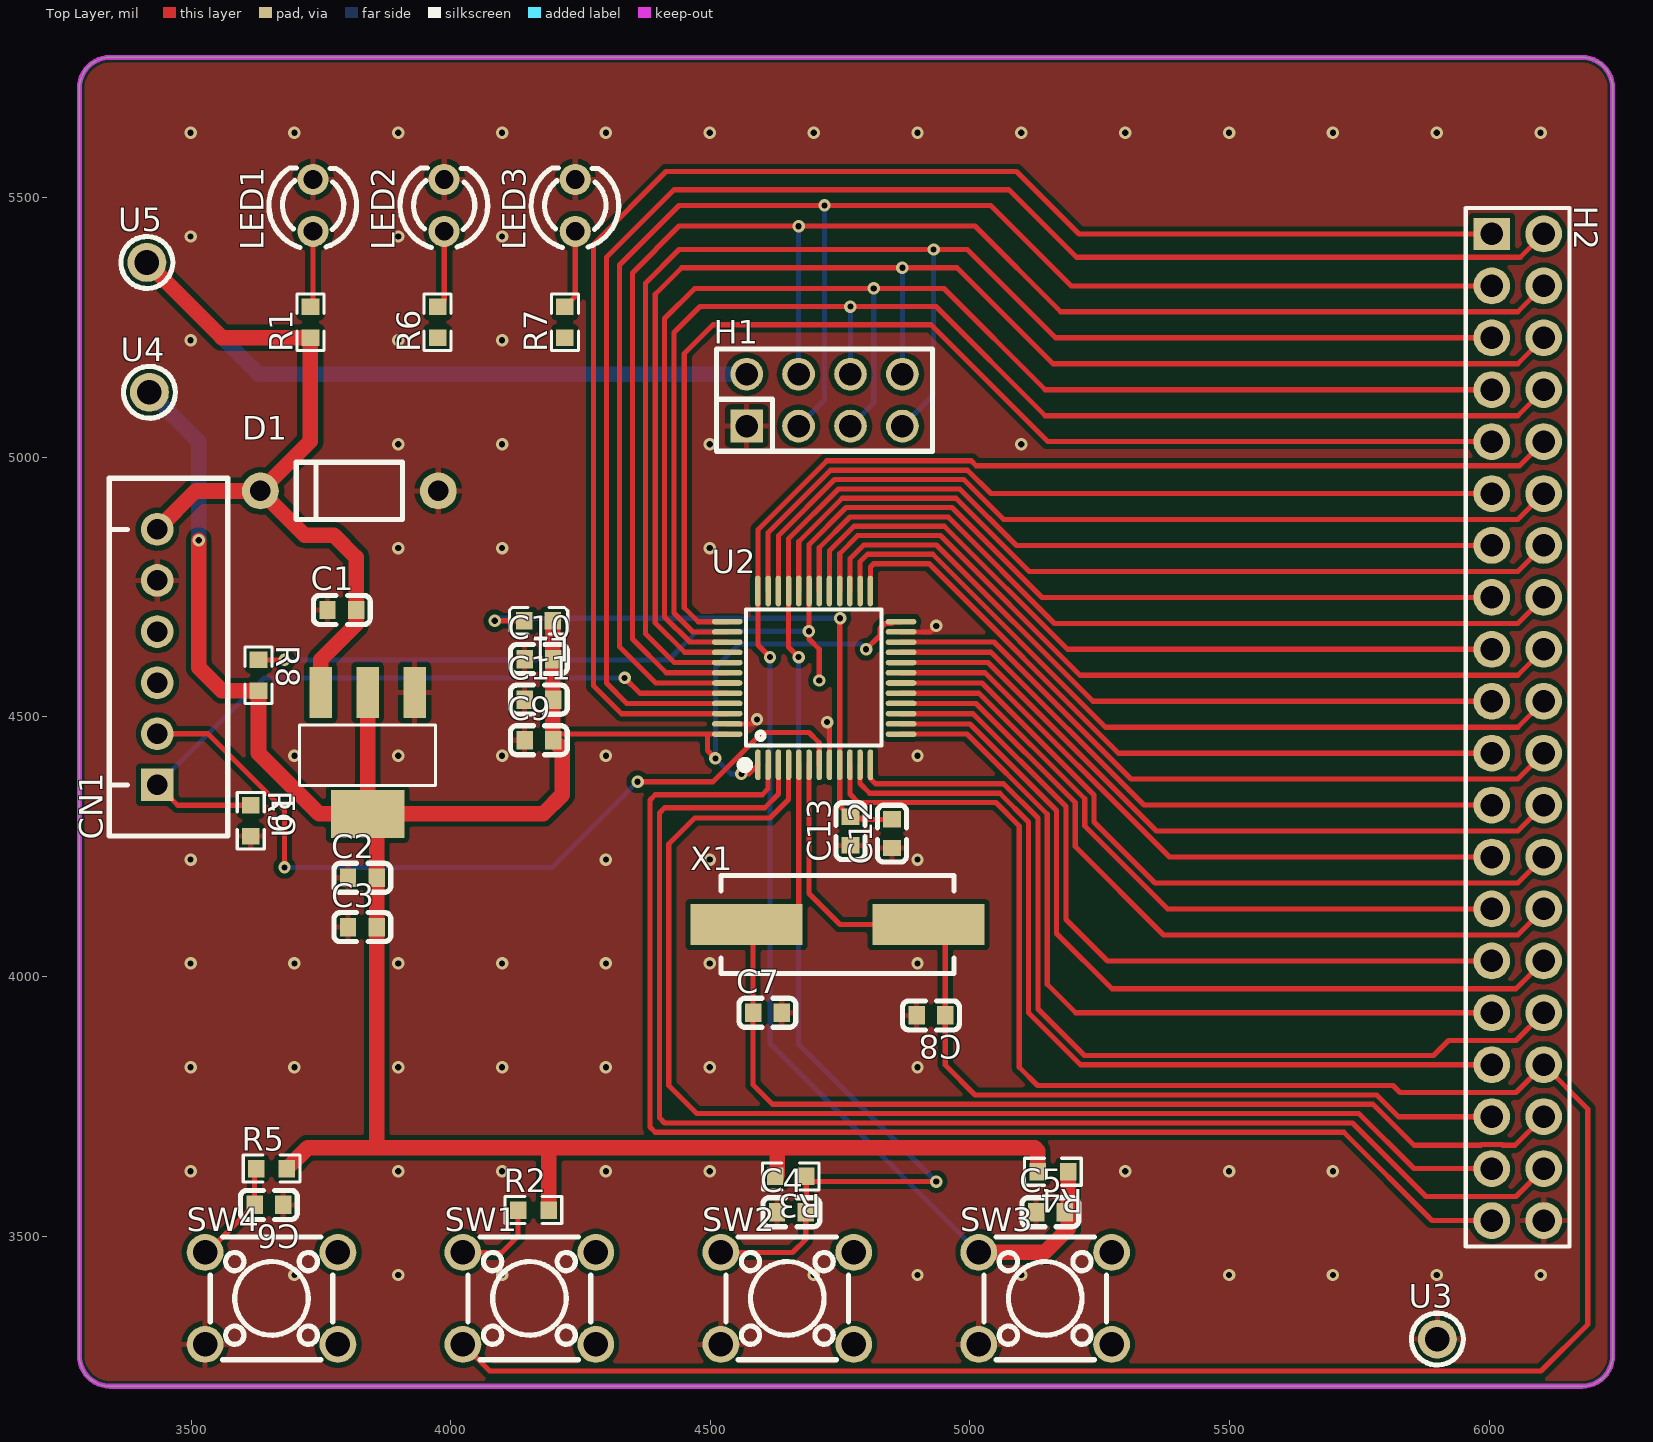
[diagram p0: Top Layer view]
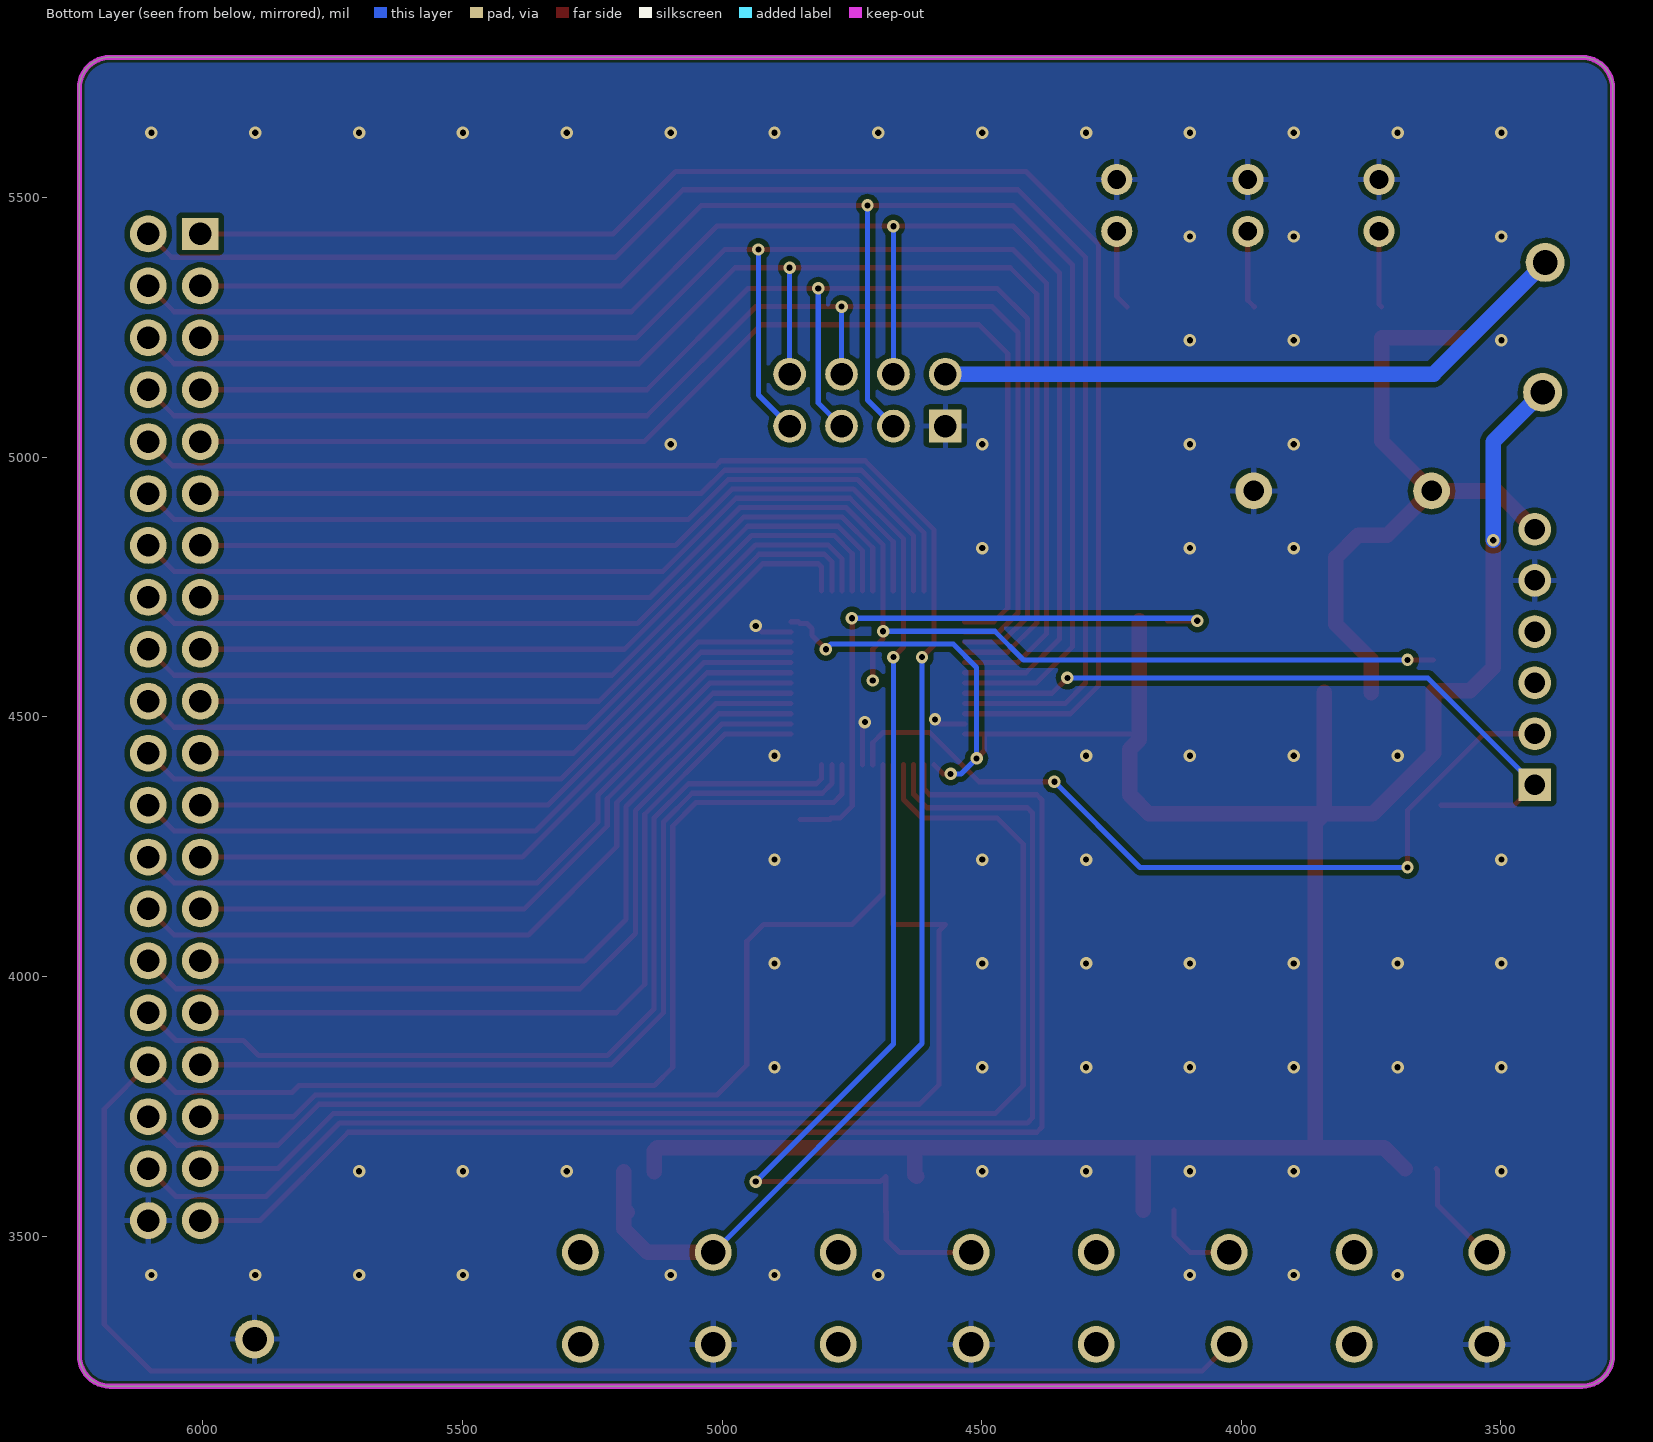
[diagram p1: Bottom Layer view, seen from below]
# Altium PCB MISC75379.pcbdoc
Units mil, origin at the board's own origin, x right, y up, seen from the top; angles counter-clockwise.
Board outline 2952.76 x 2559.06 mil, 2 copper layers (Top Layer, Bottom Layer), stack 62.206 mil thick; 40 components, 54 nets, 181 pads, 92 vias.

## Layer stack, top to bottom
Top Solder Mask Layer: solder mask 0.394, Dk 3.3
Top Layer: signal copper 1.379
Dielectric1: surface 59.449, FR4, Dk 4.5
Bottom Layer: signal copper 1.378
Bottom Solder Mask Layer: solder mask 0.394, Dk 3.3

## Board outline
3344.06,5770 ccw(c3344.06,5710.94) 3285,5710.94 3285,3270 ccw(c3344.06,3270) 3344.06,3210.94 6178.7,3210.94 ccw(c6178.7,3270) 6237.76,3270 6237.76,5710.94 ccw(c6178.7,5710.94) 6178.7,5770 3344.06,5770

## Design rules (kind name [scope] priority, off if disabled: settings)
BoardOutlineClearance copperThickness2oz_1 [All] p2 off: genericclearance=7.99 ignorepadtopadclearanceinfootprint=FALSE except(0: Arc-SplitContinuation Track-SplitContinuation SMDPad-SplitContinuation THPad-SplitContinuation Via-SplitContinuation Fill-SplitContinuation Region-SplitContinuation Poly-SplitContinuation Text-SplitContinuation Hole-SplitContinuation; 5.98: Arc-CutoutEdge SMDPad-CutoutEdge THPad-CutoutEdge Via-CutoutEdge Fill-CutoutEdge Region-CutoutEdge Text-CutoutEdge; 6.93: Hole-OutlineEdge Hole-CutoutEdge; 10: Poly-OutlineEdge Poly-CutoutEdge; 11.81: Arc-OutlineEdge Track-OutlineEdge SMDPad-OutlineEdge THPad-OutlineEdge Via-OutlineEdge Fill-OutlineEdge Region-OutlineEdge Text-OutlineEdge Track-CutoutEdge)
BoardOutlineClearance copperThickness1oz_1 [All] p4: genericclearance=8 ignorepadtopadclearanceinfootprint=FALSE except(0: Arc-SplitContinuation Track-SplitContinuation SMDPad-SplitContinuation THPad-SplitContinuation Via-SplitContinuation Fill-SplitContinuation Region-SplitContinuation Poly-SplitContinuation Text-SplitContinuation Hole-SplitContinuation; 6: SMDPad-CutoutEdge THPad-CutoutEdge Via-CutoutEdge Fill-CutoutEdge Region-CutoutEdge Text-CutoutEdge; 6.93: Hole-OutlineEdge Hole-CutoutEdge; 10: Poly-OutlineEdge Poly-CutoutEdge; 11.8: Arc-OutlineEdge Track-OutlineEdge SMDPad-OutlineEdge THPad-OutlineEdge Via-OutlineEdge Fill-OutlineEdge Region-OutlineEdge Text-OutlineEdge; 11.81: Arc-CutoutEdge Track-CutoutEdge)
Clearance copperThickness2oz [All] p1 off: gap=7.99 ignorepadtopadclearanceinfootprint=FALSE except(5.98: SMDPad-Track SMDPad-SMDPad THPad-Track SMDPad-THPad THPad-THPad Track-Via SMDPad-Via THPad-Via Via-Via Fill-Track Region-Track Fill-SMDPad Region-SMDPad Fill-THPad Region-THPad Fill-Via Region-Via Fill-Fill Fill-Region Region-Region Arc-Track Arc-SMDPad Arc-THPad Arc-Via Fill-Arc Region-Arc Arc-Arc Text-Track SMDPad-Text Text-THPad Text-Via Fill-Text Region-Text Arc-Text Text-Text; 6.93: Hole-Track Hole-SMDPad Hole-THPad Hole-Via Fill-Hole Region-Hole Hole-Arc Hole-Text; 10: Poly-Track Poly-SMDPad Poly-THPad Poly-Via Poly-Fill Poly-Region Poly-Poly Poly-Arc Poly-Text Poly-Hole)
Clearance copperThickness1oz [All] p3: gap=8 ignorepadtopadclearanceinfootprint=FALSE except(5.98: SMDPad-Track SMDPad-SMDPad THPad-Track SMDPad-THPad THPad-THPad Track-Via SMDPad-Via THPad-Via Fill-Track Region-Track Fill-SMDPad Region-SMDPad Fill-THPad Region-THPad Fill-Via Region-Via; 6: Arc-Track Arc-SMDPad Arc-THPad Arc-Via Fill-Arc Region-Arc Text-Track SMDPad-Text Text-THPad Text-Via Fill-Text Region-Text Arc-Text; 6.93: Hole-Track Hole-SMDPad Hole-THPad Hole-Via Fill-Hole Region-Hole Hole-Arc Hole-Text; 10: Poly-Track Poly-SMDPad Poly-THPad Poly-Via Poly-Fill Poly-Region Poly-Arc Poly-Text Poly-Hole)
DiffPairsRouting differentialPair [All] p1: maxlimit=6 minlimit=6 mostfreqgap=6 toplayer_minwidth=5 toplayer_prefwidth=10 toplayer_maxwidth=100 toplayer_mingap=6 toplayer_prefgap=6 toplayer_maxgap=6 bottomlayer_minwidth=5 bottomlayer_prefwidth=10 bottomlayer_maxwidth=100 bottomlayer_mingap=6 bottomlayer_prefgap=6 bottomlayer_maxgap=6 maxuncoupledlength=10
HoleToHoleClearance otherClearance [All] p1: gap=11.81 allowstackedmicrovias=TRUE
Length netLength [All] p1: minlimit=0 maxlimit=0
MatchedLengths netLengthTolerance [All] p1: tolerance=1000
PasteMaskExpansion pasteMaskExpansion [All] p1: expansion=0
PlaneConnect innerPlane [All] p1: planeconnectstyle=Relief reliefexpansion=20 reliefentries=4 reliefconductorwidth=10 reliefairgap=10
PolygonConnect copperRegion [(InNet('GND'))] p1: connectstyle=Relief reliefconductorwidth=10 reliefentries=4 polygonreliefangle="90 Angle" airgapwidth=10 via.connectstyle=Relief via.reliefconductorwidth=10 via.reliefentries=4 via.polygonreliefangle="90 Angle" via.airgapwidth=10
RoutingVias viaSize [All] p1: holewidth=12.01 width=24.02 viastyle="Through Hole" minholewidth=11.81 minwidth=19.68 maxholewidth=248.03 maxwidth=393.7
SolderMaskExpansion solderMaskExpansion [IsVia] p1: expansion=-1000 istentingtop=TRUE
SolderMaskExpansion solderMaskExpansion [All] p2: expansion=2 istentingtop=FALSE
Width copperThickness2oz_2 [All] p1 off: maxlimit=100 minlimit=8 preferedwidth=10
Width copperThickness1oz_2 [All] p2: maxlimit=100 minlimit=5 preferedwidth=10

## Components (designator, comment, footprint, x,y, rotation, side; value= is the part's Value field where it differs from the comment)
C1 "47uF" C0603 3790.35,4705.85 r0 top
C2 "47uF" C0603 3830,4190 r0 top
C3 "100nF" C0603 3830,4095 r0 top
C4 "100nF" C0603 4656.14,3546.05 r0 top
C5 "100nF" C0603 5155,3546.05 r0 top
C6 "100nF" C0603 3650,3560 r180 top
C7 "22pF" C0603 4610,3930 r0 top
C8 "22pF" C0603 4925,3925 r180 top
C9 "100nF" C0603 4170,4455 r0 top
C10 "100nF" C0603 4170,4611.24 r0 top
C11 "100nF" C0603 4170,4533.12 r0 top
C12 "1uF" C0603 4850,4275 r90 top
C13 "10nF" C0603 4770,4280 r90 top
CN1 "XH-6A" CONN-TH_6P-P2.50_XH-6A 3435,4615 r90 top
D1 "" DO_1N4007 3805,4935 r0 top
H1 "A2541HWV-2x4P" HDR-TH_8P-P2.54-V-F-R2-C4-S2.54-1 4720,5110 r0 top
H2 "2.54mm 2*20P straight pin header" HDR-TH_40P-P2.54-V-M-R2-C20-S2.54 6055,4480 r270 top
L1 "CBG160808U000T" L0603 4169.34,4685 r180 top
LED1 "" LED_TH-3mm 3735,5485 r90 top
LED2 "" LED_TH-3mm 3987.5,5485 r90 top
LED3 "" LED_TH-3mm 4240,5485 r90 top
R1 "1K" R0603 3730,5260 r90 top
R2 "10K" R0603 4159.48,3550 r0 top
R3 "10K" R0603 4655,3615 r180 top
R4 "10K" R0603 5160,3623.95 r180 top
R5 "10K" R0603 3655,3630 r0 top
R6 "330" R0603 3975,5260 r90 top
R7 "330" R0603 4220,5260 r90 top
R8 "10K" R0603 3630,4580 r270 top
R9 "10K" R0603 3615,4300 r270 top
SW1 "TS-1095-A5B2-D1" SW-TH_4P-L6.0-W6.0-P4.50-LS6.5 4151.67,3380 r0 top
SW2 "TS-1095-A5B2-D1" SW-TH_4P-L6.0-W6.0-P4.50-LS6.5 4648.33,3380 r0 top
SW3 "TS-1095-A5B2-D1" SW-TH_4P-L6.0-W6.0-P4.50-LS6.5 5145,3380 r0 top
SW4 "TS-1095-A5B2-D1" SW-TH_4P-L6.0-W6.0-P4.50-LS6.5 3655,3380 r0 top
U1 "AMS1117-3.3" SOT-223-3_L6.5-W3.4-P2.30-LS7.0-BR 3840,4430 r90 top
U2 "GD32E230C8T6" LQFP-48_L7.0-W7.0-P0.50-LS9.0-BL 4700,4575 r0 top
U3 "RH-5000" TEST-TH_BD2.54-P1.4_RED 5900.31,3301.56 r0 top
U4 "RH-5000" TEST-TH_BD2.54-P1.4_RED 3420,5125 r0 top
U5 "RH-5000" TEST-TH_BD2.54-P1.4_RED 3415,5375 r0 top
X1 "8MHz" CRYSTAL-SMD_L11.5-W4.8-LS12.7 4745,4100 r0 top

## Footprints (in the part's own frame and the unit in brackets; to place one, negate y for a bottom-side part, rotate by r counter-clockwise, add the part's x,y. Pads: shape width x height; smd on the part's side, far side on the other; paste and mask are expansions set on the pad)
C0603 [mm]
  rect 0.8x0.9 smd: 1(-0.7,0) 2(0.7,0)
  silkscreen extent -1.39,-0.71 1.39,0.71
CONN-TH_6P-P2.50_XH-6A [mm]
  rect 1.6x1.6 hole 1: 1(-6.25,0)
  round 1.6 hole 1 copper offset 0,0: 2(-3.75,0) 6(6.25,0)
  round 1.6 hole 1: 3(-1.25,0) 4(1.25,0) 5(3.75,0)
  silkscreen extent -8.75,-3.45 8.75,2.35
CRYSTAL-SMD_L11.5-W4.8-LS12.7 [mm]
  rect 5.5x2 smd: 1(-4.45,0) 2(4.45,0)
  silkscreen extent -5.7,-2.4 5.7,2.4
DO_1N4007 [mm]
  round 1.8 hole 1 paste+0 mask+0.051: 1(-4.35,0) 2(4.35,0)
  silkscreen extent -2.6,-1.4 2.6,1.4
HDR-TH_8P-P2.54-V-F-R2-C4-S2.54-1 [mm]
  rect 1.6x1.6 hole 1.1: 1(-3.81,-1.27)
  round 1.6 hole 1.1: 2(-3.81,1.27) 3(-1.27,-1.27) 4(-1.27,1.27) 5(1.27,-1.27) 6(1.27,1.27) 7(3.81,-1.27) 8(3.81,1.27)
  silkscreen extent -5.28,-2.5 5.28,2.5
HDR-TH_40P-P2.54-V-M-R2-C20-S2.54 [mm]
  rect 1.575x1.8 hole 1.1: 1(-24.13,-1.27)
  round 1.8 hole 1.1: 2(-24.13,1.27) 3(-21.59,-1.27) 4(-21.59,1.27) 5(-19.05,-1.27) 6(-19.05,1.27) 7(-16.51,-1.27) 8(-16.51,1.27) 9(-13.97,-1.27) 10(-13.97,1.27) 11(-11.43,-1.27) 12(-11.43,1.27) 13(-8.89,-1.27) 14(-8.89,1.27) 15(-6.35,-1.27) 16(-6.35,1.27) 17(-3.81,-1.27) 18(-3.81,1.27) 19(-1.27,-1.27) 20(-1.27,1.27) 21(1.27,-1.27) 22(1.27,1.27) 23(3.81,-1.27) 24(3.81,1.27) 25(6.35,-1.27) 26(6.35,1.27) 27(8.89,-1.27) 28(8.89,1.27) 29(11.43,-1.27) 30(11.43,1.27) 31(13.97,-1.27) 32(13.97,1.27) 33(16.51,-1.27) 34(16.51,1.27) 35(19.05,-1.27) 36(19.05,1.27) 37(21.59,-1.27) 38(21.59,1.27) 39(24.13,-1.27) 40(24.13,1.27)
  silkscreen extent -25.4,-2.54 25.4,2.54
L0603 [mm]
  rect 0.8x0.864 smd paste-100 mask+0.051: 1(-0.7,0) 2(0.7,0)
  silkscreen extent -1.42,-0.65 1.42,0.65
LED_TH-3mm [mil]
  round 60 hole 36 paste+0 mask+2: 1(-50,0) 2(50,0)
  silkscreen extent -81,-84 72,85
LQFP-48_L7.0-W7.0-P0.50-LS9.0-BL [mm]
  oval 0.27x1.5 smd paste+0 mask+0.05: 1(-2.75,-4.25) 2(-2.25,-4.25) 3(-1.75,-4.25) 4(-1.25,-4.25) 5(-0.75,-4.25) 6(-0.25,-4.25) 7(0.25,-4.25) 8(0.75,-4.25) 9(1.25,-4.25) 10(1.75,-4.25) 11(2.25,-4.25) 12(2.75,-4.25) 25(2.75,4.25) 26(2.25,4.25) 27(1.75,4.25) 28(1.25,4.25) 29(0.75,4.25) 30(0.25,4.25) 31(-0.25,4.25) 32(-0.75,4.25) 33(-1.25,4.25) 34(-1.75,4.25) 35(-2.25,4.25) 36(-2.75,4.25)
  oval 1.5x0.27 smd paste+0 mask+0.05: 13(4.25,-2.75) 14(4.25,-2.25) 15(4.25,-1.75) 16(4.25,-1.25) 17(4.25,-0.75) 18(4.25,-0.25) 19(4.25,0.25) 20(4.25,0.75) 21(4.25,1.25) 22(4.25,1.75) 23(4.25,2.25) 24(4.25,2.75) 37(-4.25,2.75) 38(-4.25,2.25) 39(-4.25,1.75) 40(-4.25,1.25) 41(-4.25,0.75) 42(-4.25,0.25) 43(-4.25,-0.25) 44(-4.25,-0.75) 45(-4.25,-1.25) 46(-4.25,-1.75) 47(-4.25,-2.25) 48(-4.25,-2.75)
  silkscreen extent -3.59,-4.46 3.3,3.34
R0603 [mil]
  rect 31.75x34.02 smd paste-3937.01 mask+2: 1(-29.66,0) 2(29.66,0)
  silkscreen extent -55,-26 55,26
SOT-223-3_L6.5-W3.4-P2.30-LS7.0-BR [mm]
  rect 2.5x1.1 smd: 1(2.97,-2.3) 2(2.97,0) 3(2.97,2.3)
  rect 2.34x3.6 smd: 4(-2.97,0)
  silkscreen extent -1.57,-3.33 1.37,3.33
SW-TH_4P-L6.0-W6.0-P4.50-LS6.5 [mm]
  round 1.8 hole 1.2: 1(-3.25,2.25) 2(3.25,2.25) 3(-3.25,-2.25) 4(3.25,-2.25)
  silkscreen extent -3,-3 3,3
TEST-TH_BD2.54-P1.4_RED [mm]
  round 1.9 hole 1.2: 1(0,0)
  silkscreen extent -1.27,-1.27 1.27,1.27

## Via types
v1: diameter 24.02, hole 12, Top Layer to Bottom Layer, 92 vias

## Nets (pads, with @x,y where several pads share a name; then routed paths per layer and width w, separated by ;. In a path a pad name is that pad's centre, name@x,y a point inside that pad or via, vN(x,y) a via of type N, cw(c..) or ccw(c..) an arc to the next point about the centre after c; other vN are vias at no path point)
3V3: C2.2 C3.2 C9.2 C10.2 C11.2 L1.1 R2.2 R3.2 R4.2 R5.2 R8.2 U1.2 U1.4 U2.1 U2.24 U2.48 U4.1 | length 5462.5
  Top Layer w10: C9.2 4209.29,4466.73 4494.61,4466.73 ; v1(4510,4420) 4494.61,4435.39 4494.61,4466.73 ; U2.48 4494.61,4466.73 ; v1(4560,4390) 4574.05,4390 U2.1 ; v1(4800,4630) 4826.82,4656.82 4826.82,4670.34 4836.36,4679.88 4849.88,4679.88 4853.27,4683.27 U2.24
  Top Layer w30: v1(3515,4840) 3515,4595 3559.66,4550.34 R8.2 3630,4430 3746.93,4313.07 U1.4 ; R5.2 3724.66,3670 3857.49,3670 ; U1.2 U1.4 ; R2.2 4189.14,3663.66 4195.48,3670 ; L1.1 4196.9,4455.66 C9.2 4215,4437.56 4215,4350 4178.07,4313.07 U1.4 ; R3.2 4628.78,3618.44 4628.78,3670 ; R4.2 5130.34,3664.66 5125,3670 4628.78,3670 ; U1.4 3857.56,4295.51 C2.2 C3.2 3857.56,3670.07 3857.49,3670 ; 3857.49,3670 4195.48,3670 ; 4195.48,3670 4628.78,3670
  Bottom Layer w10: v1(4560,4390) 4540,4390 v1(4510,4420) 4510,4595 4555,4640 4790,4640 v1(4800,4630)
  Bottom Layer w30: U4.1 3515,5030 v1(3515,4840)
$1N6: LED1.1 R1.2 | length 147.4
  Top Layer w10: R1.2 3735,5294.66 LED1.1
$1N17: R2.1 SW1.1 | length 169.2
  Top Layer w10: SW1.1 4098.58,3468.58 4129.82,3499.82 R2.1
$1N84: LED2.1 R6.2 | length 150.5
  Top Layer w10: R6.2 3987.5,5302.16 LED2.1
$1N86: LED3.1 R7.2 | length 153.6
  Top Layer w10: R7.2 4240,5309.66 LED3.1
$1N87: R6.1
$1N88: R7.1
+5V: C1.2 CN1.6 D1.1 H1.2 R1.1 U1.3 U5.1 | length 2709.2
  Top Layer w30: U5.1 3559.66,5230.34 R1.1 3730,5031.26 D1.1 ; CN1.6 3508.93,4935 D1.1 ; U1.3 3749.45,4609.45 3817.91,4677.91 C1.2 3817.91,4807.09 3775,4850 3718.74,4850 D1.1
  Bottom Layer w30: U5.1 3630,5160 H1.2
BOOTO: CN1.1 R9.1 U2.44 | length 1391.5
  Top Layer w10: CN1.1 3474.27,4329.66 R9.1 ; v1(4335,4575) 4364.53,4545.47 U2.44
  Bottom Layer w10: CN1.1 3641.06,4575 v1(4335,4575)
GND: C1.1 C2.1 C3.1 C4.1 C5.1 C6.1 C7.2 C8.2 C9.1 C10.1 C11.1 C12.1 C13.1 CN1.5 D1.2 H1.1 H2.40 LED1.2 LED2.2 LED3.2 R9.2 SW2.3 SW3.3 SW4.3 U1.1 U2.8 U2.23 U2.47 U3.1 | length 217.5
  Top Layer w10: U2.47 4581.42,4486.42 v1(4590,4495) ; v1(4725,4490) 4729.53,4485.47 U2.8 ; U2.23 4923.58,4663.58 v1(4935,4675)
  other v1: 3699.1,3425.04 3899.1,3425.04 4099.1,3425.04 4699.1,3425.04 4899.1,3425.04 5099.1,3425.04 5499.1,3425.04 5699.1,3425.04 5899.1,3425.04 6099.1,3425.04 3499.1,3625.04 3899.1,3625.04 4099.1,3625.04 4299.1,3625.04 4499.1,3625.04 5299.1,3625.04 5499.1,3625.04 5699.1,3625.04 3499.1,3825.04 3699.1,3825.04 3899.1,3825.04 4099.1,3825.04 4299.1,3825.04 4499.1,3825.04 4899.1,3825.04 3499.1,4025.04 3699.1,4025.04 3899.1,4025.04 4099.1,4025.04 4299.1,4025.04 4499.1,4025.04 4899.1,4025.04 3499.1,4225.04 4299.1,4225.04 4499.1,4225.04 4899.1,4225.04 3699.1,4425.04 3899.1,4425.04 4099.1,4425.04 4299.1,4425.04 4899.1,4425.04 3899.1,4825.04 4099.1,4825.04 4499.1,4825.04 3899.1,5025.04 4099.1,5025.04 4499.1,5025.04 5099.1,5025.04 3499.1,5225.04 3899.1,5225.04 4099.1,5225.04 3499.1,5425.04 3899.1,5425.04 4099.1,5425.04 3499.1,5625.04 3699.1,5625.04 3899.1,5625.04 4099.1,5625.04 4299.1,5625.04 4499.1,5625.04 4699.1,5625.04 4899.1,5625.04 5099.1,5625.04 5299.1,5625.04 5499.1,5625.04 5699.1,5625.04 5899.1,5625.04 6099.1,5625.04
KEY1: H2.34 SW1.3 U2.10 | length 4685.4
  Top Layer w10: SW1.3 4075.14,3240 6100,3240 6190,3330 6190,3745 H2.34 6051.42,3776.42 5828.58,3776.42 5815,3790 5130,3790 5095,3825 5095,4290 5050,4335 4785,4335 4768.9,4351.1 U2.10
KEY2: C4.2 H2.13 R3.1 SW2.1 U2.33 | length 3344.8
  Top Layer w10: SW2.1 4658.58,3468.58 4683.7,3493.7 C4.2 4684.66,3547.01 R3.1 4694.66,3605 v1(4935,3605) ; v1(4670,4615) 4650.79,4634.21 U2.33 4650.79,4843.07 4746.72,4939 4980.57,4939 5089.57,4830 H2.13
  Bottom Layer w10: v1(4670,4615) 4670,3870 v1(4935,3605)
KEY3: C5.2 H2.10 R4.1 SW3.1 U2.36 | length 3470.3
  Top Layer w10: v1(4615,4615) 4591.73,4638.27 U2.36 4591.73,4860.38 4724.35,4993 5002.94,4993 5012.36,4983.58 6058.58,4983.58 H2.10
  Top Layer w30: SW3.1 5143.58,3468.58 5189.66,3514.66 C5.2@5189.66,3553.15 ; C5.2 C5.2@5189.66,3553.15 ; R4.1 C5.2@5189.66,3553.15
  Bottom Layer w10: v1(4615,4615) 4615,3870.63 SW3.1
KEY4: C6.2 R5.1 SW4.1 | length 204.5
  Top Layer w10: SW4.1 3531.02,3468.58 C6.2 3622.44,3627.1 R5.1
LED1: H2.17 U2.29 | length 1470.8
  Top Layer w10: U2.29 4729.53,4819.99 4776.54,4867 4950.75,4867 5187.75,4630 H2.17
LED2: H2.1 U2.46 | length 2967.7
  Top Layer w10: U2.46 4328.9,4506.1 4275,4560 4275,5410 4415,5550 5090,5550 5210,5430 H2.1
NRST: CN1.2 U2.7 | length 1604.3
  Top Layer w10: CN1.2 3532.65,4467.35 3680,4320 v1(3680,4210) ; v1(4360,4375) 4505,4375 4600,4470 4690,4470 4709.84,4450.16 U2.7
  Bottom Layer w10: v1(3680,4210) 4195,4210 v1(4360,4375)
OSC_IN: C7.1 H2.36 U2.5 X1.1 | length 2316.8
  Top Layer w10: U2.5 4670.47,4100 X1.1 4582.44,4087.36 C7.1 4582.44,3791.56 4620,3754 5776,3754 5855,3675 5984.36,3675 5985.77,3676.42 6024.23,3676.42 6025.64,3675 6050,3675 H2.36
OSC_OUT: C8.1 H2.35 U2.6 X1.2 | length 1880.3
  Top Layer w10: U2.6 4690.16,4159.84 4750,4100 X1.2 4952.56,4067.64 C8.1 4952.56,3829.44 5010,3772 5783.46,3772 5825.46,3730 H2.35
PA1: H2.33 U2.11 | length 1692.2
  Top Layer w10: U2.11 4788.58,4371.42 4807,4353 5057.46,4353 5113,4297.46 5113,3930 5213,3830 H2.33
PA2: H2.32 U2.12 | length 1793.5
  Top Layer w10: U2.12 4808.27,4380.8 4818.07,4371 5064.91,4371 5131,4304.91 5131,3937.46 5220.46,3848 5893,3848 5921.42,3876.42 6051.42,3876.42 H2.32
PA3: H2.31 U2.13 | length 1551.8
  Top Layer w10: U2.13 4994.64,4466.73 5149,4312.37 5149,3985 5204,3930 H2.31
PA4: H2.30 U2.14 | length 1609.9
  Top Layer w10: U2.14 5000.4,4486.42 5167,4319.82 5167,4083 5273.58,3976.42 6051.42,3976.42 H2.30
PA5: H2.29 U2.15 | length 1462.2
  Top Layer w10: U2.15 5006.18,4506.1 5185,4327.28 5185,4110 5265,4030 H2.29
PA6: H2.28 U2.16 | length 1492.7
  Top Layer w10: U2.16 5011.95,4525.79 5203,4334.74 5203,4250 5373,4080 6055,4080 H2.28
PA7: H2.27 U2.17 | length 1340.3
  Top Layer w10: U2.17 5017.72,4545.47 5221,4342.19 5221,4290 5381,4130 H2.27
PA9: H2.16 U2.30 | length 1608.8
  Top Layer w10: U2.30 4709.84,4825.75 4769.09,4885 4958.21,4885 5163.21,4680 6055,4680 H2.16
PA10: H2.15 R8.1 U2.31 | length 2768.8
  Top Layer w10: R8.1 v1(3680,4609.66) ; v1(4710,4570) 4710,4630 4690.16,4649.84 U2.31 4690.16,4831.53 4761.63,4903 4965.66,4903 5138.66,4730 H2.15
  Bottom Layer w10: v1(3680,4609.66) 4419.66,4609.66 4475,4665 v1(4690,4665)
PA11: H2.14 U2.32 | length 1643.3
  Top Layer w10: U2.32 4670.47,4837.29 4754.18,4921 4973.12,4921 5114.12,4780 6055,4780 H2.14
PA13: H2.12 U2.34 | length 1677.8
  Top Layer w10: U2.34 4631.1,4848.84 4739.26,4957 4988.03,4957 5065.03,4880 6055,4880 H2.12
PA14: H2.9 U2.37 | length 2254.7
  Top Layer w10: U2.37 4476.73,4683.27 4450,4710 4450,5200 4505,5255 4925,5255 5150,5030 H2.9
PA15: H1.6 H2.8 U2.38 | length 2591.2
  Top Layer w10: U2.38 4466.42,4663.58 4430,4700 4430,5240 4480,5290 v1(4770,5290) 4935,5290 5145,5080 6055,5080 H2.8
  Bottom Layer w10: H1.6 v1(4770,5290)
PB0: H2.26 U2.18 | length 1448.5
  Top Layer w10: U2.18 5023.49,4565.16 5239,4349.65 5239,4297.46 5356.46,4180 6055,4180 H2.26
PB1: H2.25 U2.19 | length 1284.7
  Top Layer w10: U2.19 5029.26,4584.84 5384.1,4230 H2.25
PB2: H2.24 U2.20 | length 1392.8
  Top Layer w10: U2.20 5035.03,4604.53 5359.56,4280 6055,4280 H2.24
PB3: H1.5 H2.7 U2.39 | length 2696.7
  Top Layer w10: U2.39 4460.64,4643.9 4412,4692.54 4412,5267 4470,5325 v1(4815,5325) 4950,5325 5145,5130 H2.7
  Bottom Layer w10: H1.5 4815,5105 v1(4815,5325)
PB4: H1.8 H2.6 U2.40 | length 2829.7
  Top Layer w10: U2.40 4450.79,4624.21 4394,4681 4394,5314 4445,5365 v1(4870,5365) 4975,5365 5160,5180 6055,5180 H2.6
  Bottom Layer w10: H1.8 v1(4870,5365)
PB5: H1.7 H2.5 U2.41 | length 2947.8
  Top Layer w10: U2.41 4430.47,4604.53 4375,4660 4375,5335 4440,5400 v1(4930,5400) 4995,5400 5165,5230 H2.5
  Bottom Layer w10: H1.7 4930,5120 v1(4930,5400)
PB6: H1.4 H2.4 U2.42 | length 3081
  Top Layer w10: U2.42 4415.16,4584.84 4350,4650 4350,5355 4440,5445 v1(4670,5445) 5010,5445 5175,5280 6055,5280 H2.4
  Bottom Layer w10: H1.4 v1(4670,5445)
PB7: H1.3 H2.3 U2.43 | length 3209.2
  Top Layer w10: U2.43 4394.84,4565.16 4325,4635 4325,5370 4440,5485 v1(4720,5485) 5040,5485 5195,5330 H2.3
  Bottom Layer w10: H1.3 4720,5110 v1(4720,5485)
PB8: H2.2 U2.45 | length 3000.3
  Top Layer w10: U2.45 4339.21,4525.79 4300,4565 4300,5385 4430,5515 5075,5515 5205,5385 6060,5385 H2.2
PB10: H2.23 U2.21 | length 1259.5
  Top Layer w10: U2.21 5040.8,4624.21 5335.01,4330 H2.23
PB11: H2.22 U2.22 | length 1367.7
  Top Layer w10: U2.22 5046.57,4643.9 5310.47,4380 6055,4380 H2.22
PB12: H2.21 U2.25 | length 1396.7
  Top Layer w10: U2.25 4808.27,4788.27 4815,4795 4920.93,4795 5285.93,4430 H2.21
PB13: H2.20 U2.26 | length 1537.3
  Top Layer w10: U2.26 4788.58,4798.58 4803,4813 4928.38,4813 5261.38,4480 6055,4480 H2.20
PB14: H2.19 U2.27 | length 1433.9
  Top Layer w10: U2.27 4768.9,4804.36 4795.54,4831 4935.84,4831 5236.84,4530 H2.19
PB15: H2.18 U2.28 | length 1574.2
  Top Layer w10: U2.28 4749.21,4814.21 4784,4849 4943.29,4849 5212.29,4580 6055,4580 H2.18
PC13: H2.39 U2.2 | length 2608.1
  Top Layer w10: U2.2 4611.42,4361.42 4600,4350 4394,4350 4384,4340 4384,3710 4394,3700 5720,3700 5890,3530 H2.39
PC14: H2.38 U2.3 | length 2675.6
  Top Layer w10: U2.3 4631.1,4351.1 4605,4325 4412,4325 4402,4315 4402,3728 4412,3718 5736.86,3718 5878.44,3576.42 6051.42,3576.42 H2.38
PC15: H2.37 U2.4 | length 2449.5
  Top Layer w10: U2.4 4650.79,4340.79 4615,4305 4470,4305 4420,4255 4420,3790 4474,3736 5749,3736 5855,3630 H2.37
PF6: H2.11 U2.35 | length 1574.4
  Top Layer w10: U2.35 4611.42,4854.61 4731.81,4975 4995.48,4975 5040.48,4930 H2.11
USART_RX: CN1.4
USART_TX: CN1.3
VDDA: C12.2 C13.2 L1.2 U2.9 | length 1197.3
  Top Layer w10: v1(4085,4685) L1.2 ; v1(4750,4690) 4749.21,4689.21 U2.9 4749.21,4328.35 C13.2 4772.56,4305 4790,4305 4792.44,4302.56 C12.2
  Bottom Layer w10: v1(4085,4685) 4090,4690 v1(4750,4690)
pads on no net: SW1.2 SW1.4 SW2.2 SW2.4 SW3.2 SW3.4 SW4.2 SW4.4

## Polygon pours and split planes (outlines as drawn)
GND on Top Layer (solid, remove dead copper, pour order 0): 3115,5970 3115,3000 6515,3000 6515,5970
GND on Bottom Layer (solid, remove dead copper, pour order 2): 3000,5985 3000,3000 6575,3000 6575,5985

## Keep-outs
Board Outline Layer:
  the board outline again, w10